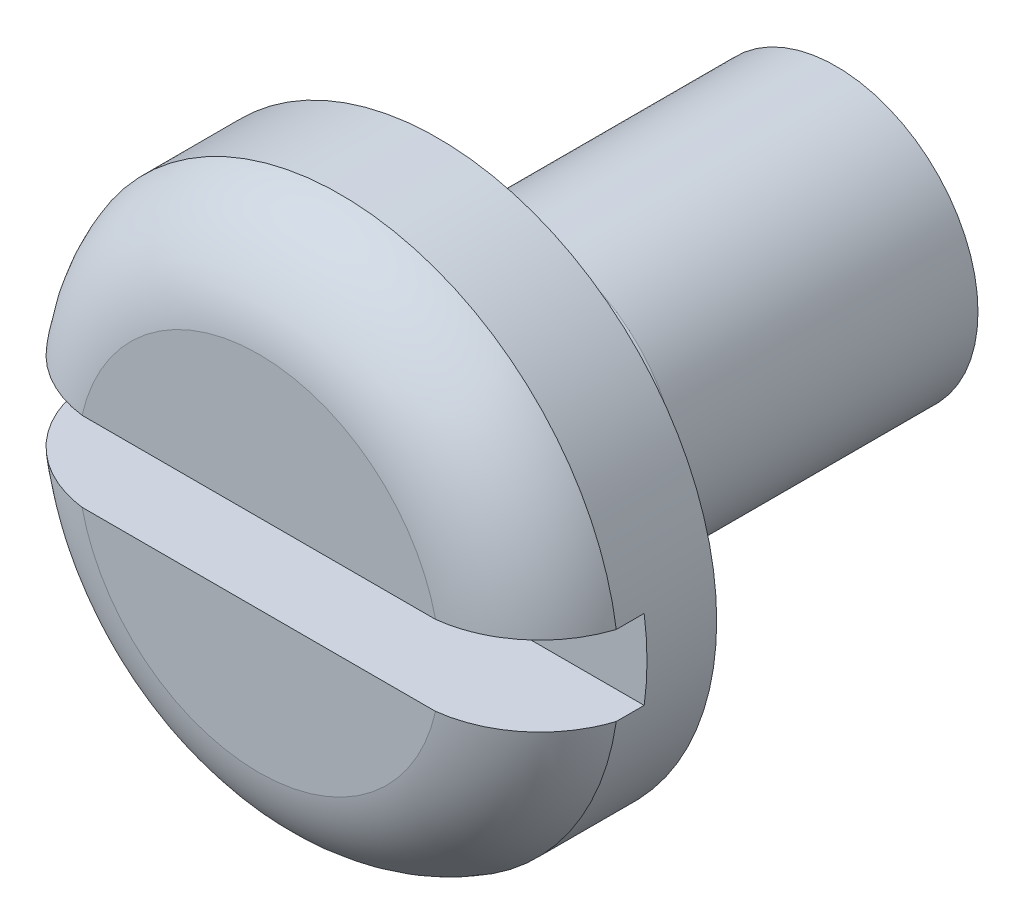
SolidWorks part; units mm, degrees
ref_plane "Front plane" through (0, 0, 0) normal (0, 0, 1) x (1, 0, 0)
ref_plane "Top plane" through (0, 0, 0) normal (0, 1, 0) x (1, 0, 0)
ref_plane "Right plane" through (0, 0, 0) normal (1, 0, 0) x (0, 0, -1)
sketch "Sketch 1" plane through (0, 0, 0) normal (0, 0, 1) x (1, 0, 0)
  circle A0 centre (0, 0) radius 2.8
  dimension "D1" = 5.6
extrude "Boss-Extrude 1" add sketch "Sketch 1" along normal blind 1.8
sketch "Sketch 3" plane through (0, 0, 0) normal (0, 1, 0) x (1, 0, 0)
  line L0 (0, 0) -> (1.475, 0)
  line L1 (0, 0) -> (0, 1.2132) construction
  line L2 (0, 0) -> (0, 0.1)
  line L3 (0, 0.1) -> (1.375, 0.1)
  arc A0 (1.375, 0.1) -> (1.475, 0) centre (2.048, 0.673) ccw
  dimension "D1" = 1.475
  dimension "D2" = 1.375
  dimension "D3" = 0.1
revolve "Revolve 1" add sketch "Sketch 3" angle 360 about L1
sketch "Sketch 4" plane through (0, 0, -0.1) normal (0, 0, -1) x (-1, 0, 0)
  circle A0 centre (0, 0) radius 1.375
extrude "Boss-Extrude 2" add sketch "Sketch 4" along normal blind 0.7
sketch "Sketch 5" plane through (0, 0, 0) normal (0, 1, 0) x (1, 0, 0)
  line L0 (0, 0) -> (0, 1.6696) construction
  line L3 (0, 0.8) -> (1.375, 0.8)
  line L4 (1.375, 0.8) -> (1.425, 1)
  line L5 (1.425, 1) -> (0, 1)
  line L6 (0, 1) -> (0, 0.8)
  point P5 (0, 0.8)
  dimension "D1" = 1.425
  dimension "D2" = 0.2
revolve "Revolve 2" add sketch "Sketch 5" angle 360 about L0
sketch "Sketch 6" plane through (0, 0, -1) normal (0, 0, -1) x (-1, 0, 0)
  circle A0 centre (0, 0) radius 1.425
  dimension "D1" = 2.85
extrude "Boss-Extrude 3" add sketch "Sketch 6" along normal blind 3
ref_plane "Reference plane 1" through (-2.8, 0, 0) normal (-1, 0, 0) x (0, 0, 1)
sketch "Sketch 7" plane through (0, 0, 0) normal (0, 1, 0) x (1, 0, 0)
  line L0 (1.82, -1.8) -> (2.8, -1.8)
  line L1 (0, 0.1168) -> (0, -3.2404) construction
  line L3 (-2.8, -1.8) -> (2.8, -1.8) construction
  line L6 (2.8, -1.8) -> (2.8, 0) construction
  line L7 (2.8, -1.8) -> (2.8, -0.98)
  arc A2 (2.8, -0.98) -> (1.82, -1.8) centre (1.6691, -0.624) cw
revolve "Cut-Revolve 3" cut sketch "Sketch 7" angle 360 about L1
sketch "Sketch 8" plane through (-2.8, 0, 0) normal (-1, 0, 0) x (0, 0, 1)
  line L0 (-0.0554, 0) -> (2.9813, 0) construction
  line L3 (0.7, -0.4) -> (0.7, 0.4)
  line L7 (0.7, -0.4) -> (2.0682, -0.4)
  line L8 (2.0682, -0.4) -> (2.0682, 0.4)
  line L9 (2.0682, 0.4) -> (0.7, 0.4)
extrude "Cut-Extrude 1" cut sketch "Sketch 8" against normal through all
